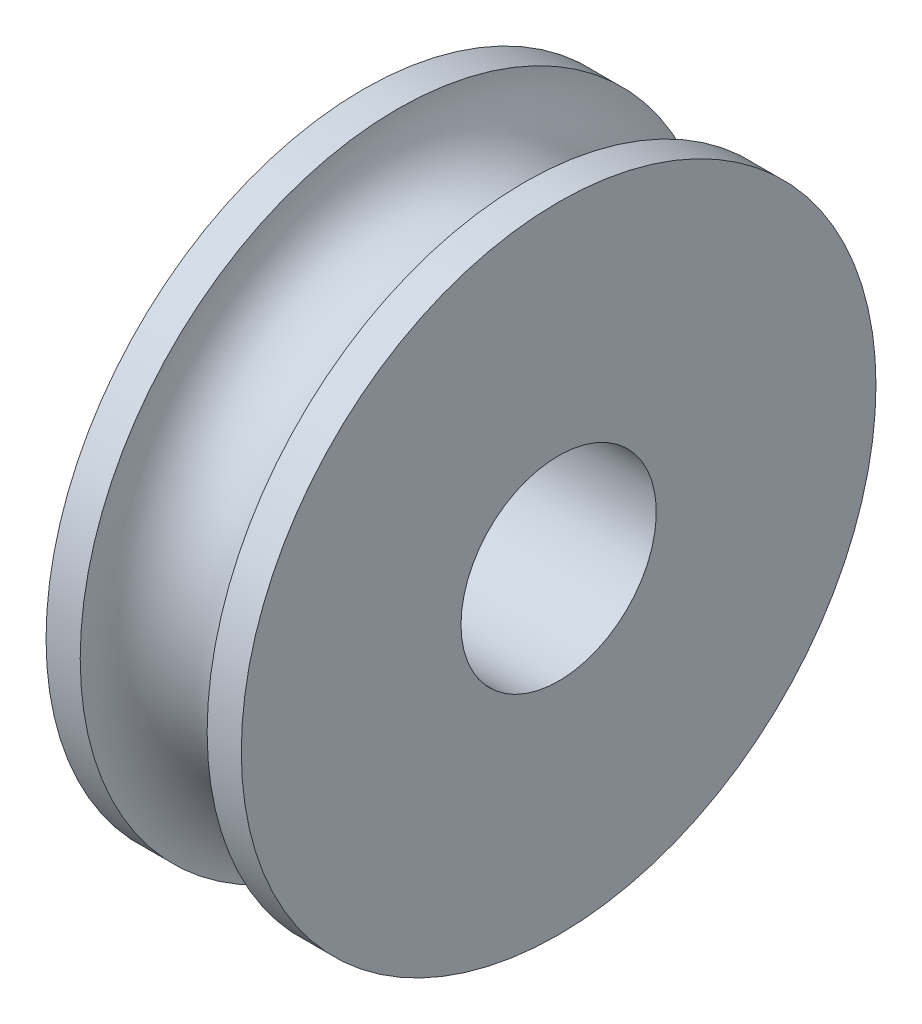
SolidWorks part; units mm, degrees
material "1060 Alloy"
ref_plane "Front Plane" through (0, 0, 0) normal (0, 0, 1) x (1, 0, 0)
ref_plane "Top Plane" through (0, 0, 0) normal (0, 1, 0) x (1, 0, 0)
ref_plane "Right Plane" through (0, 0, 0) normal (1, 0, 0) x (0, 0, -1)
sketch "Sketch1" plane through (0, 0, 0) normal (0, 1, 0) x (1, 0, 0)
  line L0 (0, 0) -> (4, 0) construction
  line L1 (0, 2) -> (4, 2)
  line L2 (4, 2) -> (4, 6.5)
  line L3 (4, 6.5) -> (3.3, 6.5)
  line L4 (0, 2) -> (0, 6.5)
  line L5 (0, 6.5) -> (0.7, 6.5)
  arc A0 (0.7, 6.5) -> (3.3, 6.5) centre (2, 6.5) ccw
  dimension "D5" = 1.3
  dimension "D1" = 4
  dimension "D2" = 4
  dimension "D3" = 13
  dimension "D4" = 0.7
revolve "Revolve1" add sketch "Sketch1" angle 360 about L0
